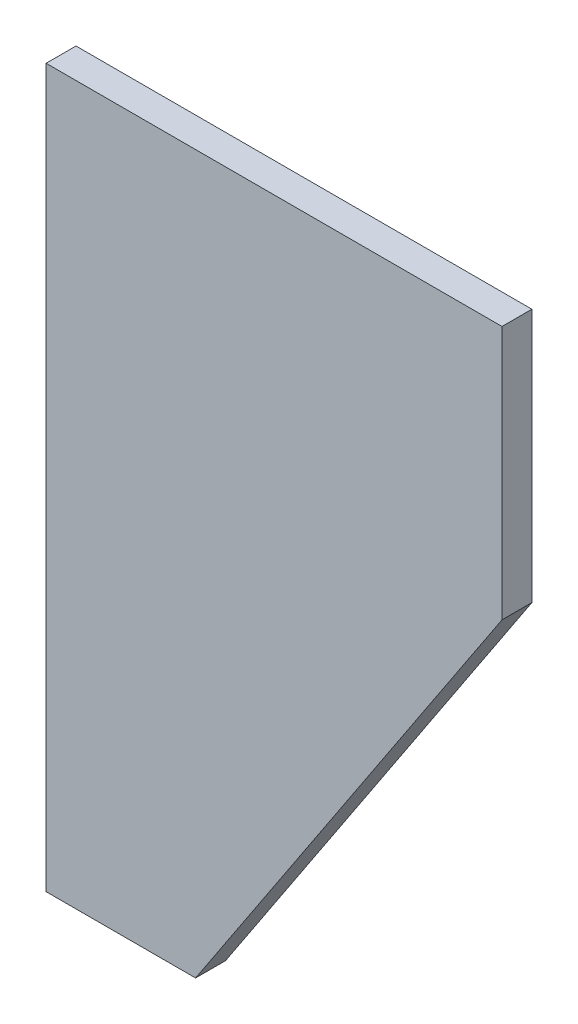
SolidWorks part; units mm, degrees
material "普通碳钢"
ref_plane "前视基准面" through (0, 0, 0) normal (0, 0, 1) x (1, 0, 0)
ref_plane "上视基准面" through (0, 0, 0) normal (0, 1, 0) x (1, 0, 0)
ref_plane "右视基准面" through (0, 0, 0) normal (1, 0, 0) x (0, 0, -1)
sketch "草图1" plane through (0, 0, 0) normal (0, 0, 1) x (1, 0, 0)
  line L0 (0, 0) -> (30.5, 0)
  line L1 (30.5, 0) -> (30.5, -17)
  line L2 (30.5, -17) -> (10, -48)
  line L3 (10, -48) -> (0, -48)
  line L4 (0, -48) -> (0, 0)
  dimension "D1" = 30.5
  dimension "D2" = 48
  dimension "D3" = 17
  dimension "D4" = 10
extrude "凸台-拉伸1" add sketch "草图1" along normal blind 2
